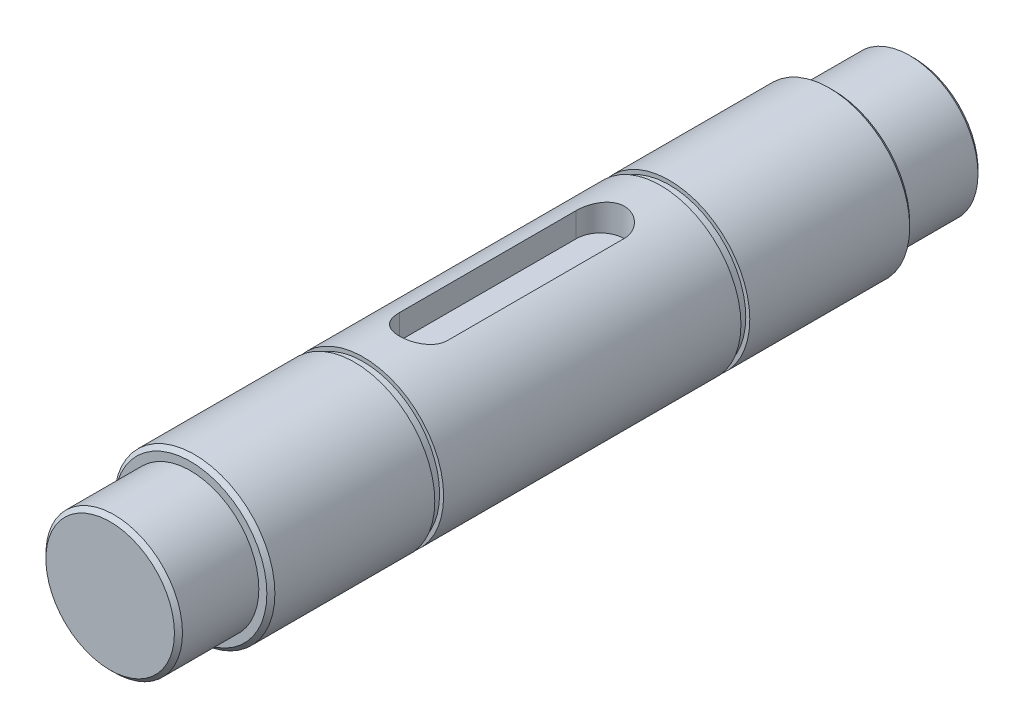
from build123d import *

# Parameters (mm, degrees)
SKETCH_1_R          = 10
EXTRUDE_1_DEPTH     = 40
SKETCH_2_R          = 8.5
EXTRUDE_2_DEPTH     = 10
CUT_EXTRUDE_START   = 1.1
SKETCH_4_R          = 10
SKETCH_4_R_2        = 9.5
CUT_EXTRUDE_1_DEPTH = 1.1
CHAMFER_1_SIZE      = 0.5
CUT_EXTRUDE_2_DEPTH = 3.5


with BuildPart() as part:
    # 草图1 → 凸台-拉伸1 (new, symmetric)
    with BuildSketch(Plane.XY):
        Circle(SKETCH_1_R)
    extrude(amount=EXTRUDE_1_DEPTH, both=True)

    # 草图2 → 凸台-拉伸2 (add)
    with BuildSketch(Plane.XY.offset(40)):
        Circle(SKETCH_2_R)
    extrude_2 = extrude(amount=EXTRUDE_2_DEPTH)

    # 草图4 → 切除-拉伸1 (cut)
    with BuildSketch(Plane.XY.offset(18.5).offset(CUT_EXTRUDE_START)):
        Circle(SKETCH_4_R)
        Circle(SKETCH_4_R_2, mode=Mode.SUBTRACT)
    cut_extrude_1 = extrude(amount=-CUT_EXTRUDE_1_DEPTH, mode=Mode.SUBTRACT)

    # 镜向1: 凸台-拉伸2, 切除-拉伸1 across plane
    add(extrude_2.mirror(Plane.XY))
    add(cut_extrude_1.mirror(Plane.XY), mode=Mode.SUBTRACT)

    # 倒角1
    chamfer_1_edges = [part.edges().sort_by_distance(p)[0] for p in [
        (-8.5, 0, -50),
        (-10, 0, -40),
        (-10, 0, 40),
        (-8.5, 0, 50),
    ]]
    chamfer(chamfer_1_edges, length=CHAMFER_1_SIZE)

    # 草图5 → 切除-拉伸2 (cut)
    with BuildSketch(Plane(origin=(0, 10, 0), x_dir=(1, 0, 0), z_dir=(0, 1, 0))):
        with BuildLine():
            Line((3, 11), (3, -11))
            ThreePointArc((3, -11), (0, -14), (-3, -11))
            Line((-3, -11), (-3, 11))
            ThreePointArc((-3, 11), (0, 14), (3, 11))
        make_face()
    extrude(amount=-CUT_EXTRUDE_2_DEPTH, mode=Mode.SUBTRACT)


solid = part.part
